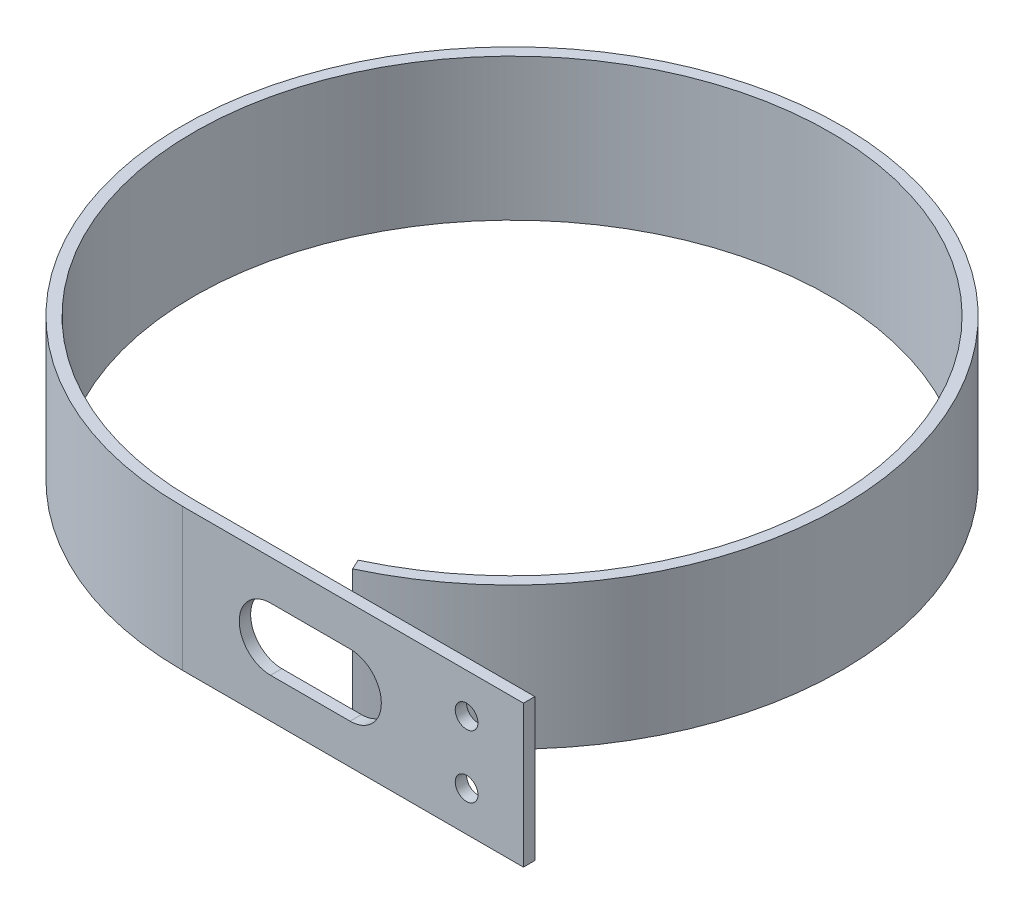
from build123d import *

# Parameters (mm, degrees)
EXTRUDE_1_DEPTH     = 12.5
SKETCH_3_R          = 2
CUT_EXTRUDE_1_DEPTH = 2


with BuildPart() as part:
    # 草图1 → 拉伸-薄壁1 (new, symmetric)
    with BuildSketch(Plane(origin=(0, 0, 0), x_dir=(1, 0, 0), z_dir=(0, 1, 0))):
        with BuildLine():
            ThreePointArc((23.666622657, -50.753236074), (-12.120618381, 54.672576399), (0, -56))
            Line((0, -56), (60, -56))
            Line((60, -56), (60, -58))
            Line((60, -58), (0, -58))
            ThreePointArc((0, -58), (-12.553497608, 56.625168413), (24.511859181, -52.565851648))
            Line((24.511859181, -52.565851648), (23.666622657, -50.753236074))
        make_face()
    extrude(amount=EXTRUDE_1_DEPTH, both=True)

    # 草图3 → 切除-拉伸1 (cut)
    with BuildSketch(Plane.XY.offset(58)):
        with Locations((50, 5.5)):
            Circle(SKETCH_3_R)
        with Locations(Location((50, -5.5, 0), (0, 0, 180))):
            Circle(SKETCH_3_R)
        with BuildLine():
            Line((15.5, 5.5), (29.5, 5.5))
            ThreePointArc((29.5, 5.5), (35, 0), (29.5, -5.5))
            Line((29.5, -5.5), (15.5, -5.5))
            ThreePointArc((15.5, -5.5), (10, 0), (15.5, 5.5))
        make_face()
    extrude(amount=-CUT_EXTRUDE_1_DEPTH, mode=Mode.SUBTRACT)


solid = part.part
